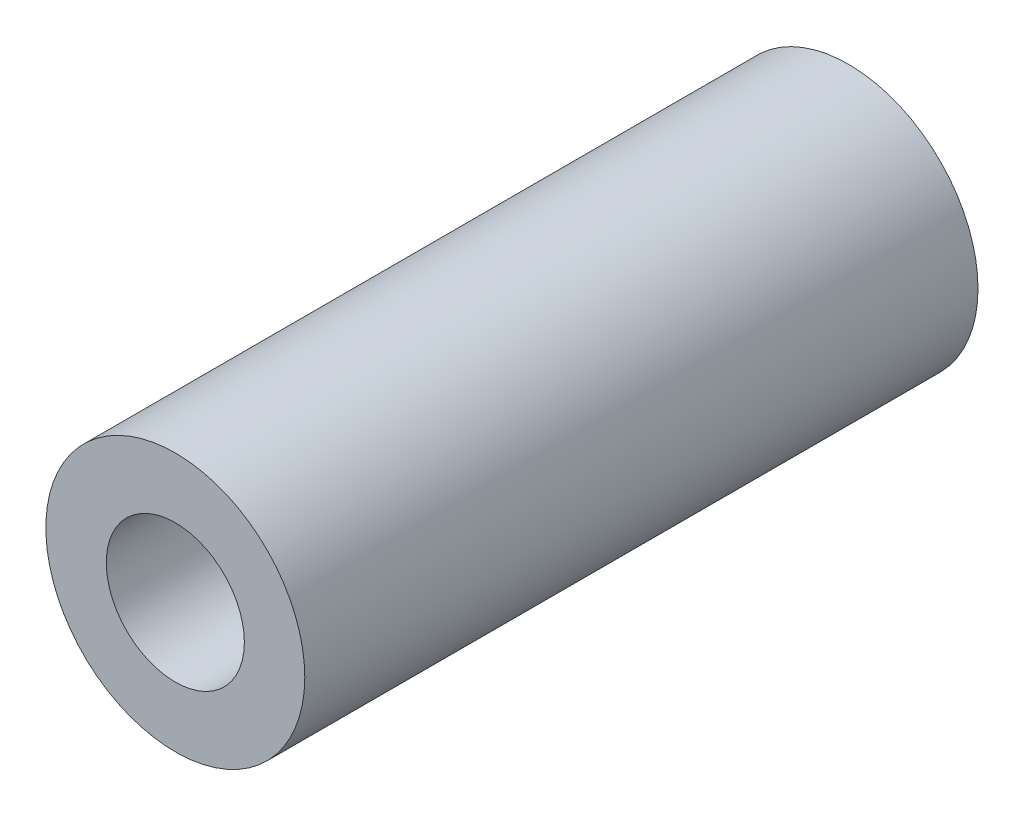
from build123d import *

# Parameters (mm, degrees)
SKETCH1_R           = 7.5
SKETCH1_R_2         = 4
BOSS_EXTRUDE1_DEPTH = 39


with BuildPart() as part:
    # Sketch1 → Boss-Extrude1 (new body)
    with BuildSketch(Plane.XY):
        Circle(SKETCH1_R)
        Circle(SKETCH1_R_2, mode=Mode.SUBTRACT)
    extrude(amount=BOSS_EXTRUDE1_DEPTH)


solid = part.part
